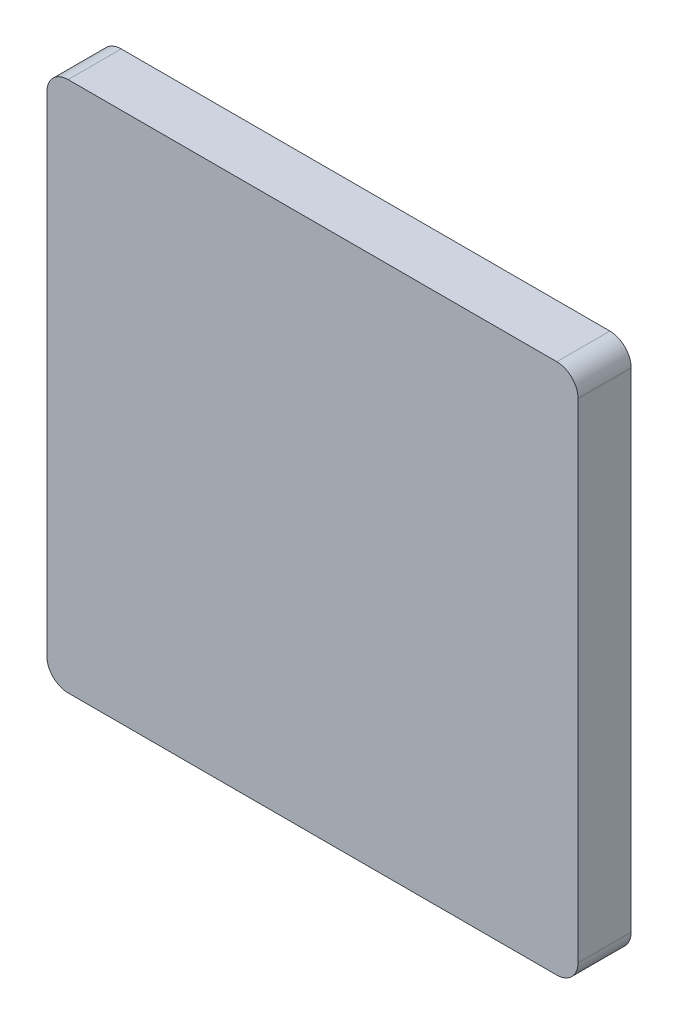
SolidWorks part; units mm, degrees
material "Q235"
ref_plane "Front Plane" through (0, 0, 0) normal (0, 0, 1) x (1, 0, 0)
ref_plane "Top Plane" through (0, 0, 0) normal (0, 1, 0) x (1, 0, 0)
ref_plane "Right Plane" through (0, 0, 0) normal (1, 0, 0) x (0, 0, -1)
sketch "Sketch1" plane through (0, 0, 0) normal (0, 0, 1) x (1, 0, 0)
  line L1 (-30, -30) -> (30, -30)
  line L2 (-30, -30) -> (-30, 30)
  line L3 (-30, 30) -> (30, 30)
  line L4 (30, -30) -> (30, 30)
  line L5 (-30, -30) -> (30, 30) construction
  line L6 (-30, 30) -> (30, -30) construction
  line L7 (-26, -26) -> (26, -26)
  line L8 (-26, -26) -> (-26, 26)
  line L9 (-26, 26) -> (26, 26)
  line L10 (26, -26) -> (26, 26)
  line L11 (-26, -26) -> (26, 26) construction
  line L12 (-26, 26) -> (26, -26) construction
  point P0 (0, 0)
  point P5 (0, 0)
  dimension "D1" = 4
  dimension "D2" = 60
  dimension "D3" = 60
extrude "Boss-Extrude1" add sketch "Sketch1" along normal blind 400
fillet "Fillet1" radius 6 4 edges at (30, -30, 200) (-30, -30, 200) (30, 30, 200) (-30, 30, 200)
fillet "Fillet2" radius 3 4 edges at (26, -26, 200) (-26, -26, 200) (26, 26, 200) (-26, 26, 200)
sketch "Sketch2" plane through (0, 0, 0) normal (0, 0, -1) x (-1, 0, 0)
  line L0 (-26, -23) -> (-26, 23) construction
  line L1 (-23, 26) -> (23, 26) construction
  line L2 (26, 23) -> (26, -23) construction
  line L3 (23, -26) -> (-23, -26) construction
  line L4 (-26, -23) -> (-26, 23) construction
  line L5 (-23, 26) -> (23, 26) construction
  line L6 (26, 23) -> (26, -23) construction
  line L7 (23, -26) -> (-23, -26) construction
  line L8 (25, 23) -> (25, -23)
  line L9 (-23, 25) -> (23, 25)
  line L10 (-25, -23) -> (-25, 23)
  line L11 (23, -25) -> (-23, -25)
  arc A0 (-26, -23) -> (-23, -26) centre (-23, -23) ccw construction
  arc A1 (-23, 26) -> (-26, 23) centre (-23, 23) ccw construction
  arc A2 (26, 23) -> (23, 26) centre (23, 23) ccw construction
  arc A3 (23, -26) -> (26, -23) centre (23, -23) ccw construction
  arc A4 (-26, -23) -> (-23, -26) centre (-23, -23) ccw construction
  arc A5 (-23, 26) -> (-26, 23) centre (-23, 23) ccw construction
  arc A6 (26, 23) -> (23, 26) centre (23, 23) ccw construction
  arc A7 (23, -26) -> (26, -23) centre (23, -23) ccw construction
  arc A8 (23, -25) -> (25, -23) centre (23, -23) ccw
  arc A9 (25, 23) -> (23, 25) centre (23, 23) ccw
  arc A10 (-23, 25) -> (-25, 23) centre (-23, 23) ccw
  arc A11 (-25, -23) -> (-23, -25) centre (-23, -23) ccw
  dimension "D1" = 1
extrude "Boss-Extrude2" add sketch "Sketch2" along normal blind 5 separate body
sketch "Sketch4" plane through (0, 0, 0) normal (0, 0, -1) x (-1, 0, 0)
  line L0 (26, 23) -> (26, -23) construction
  line L1 (-23, 26) -> (23, 26) construction
  line L2 (-26, -23) -> (-26, 23) construction
  line L3 (23, -26) -> (-23, -26) construction
  line L4 (-30, 24) -> (-30, -24)
  line L5 (-24, -30) -> (24, -30)
  line L6 (30, -24) -> (30, 24)
  line L7 (24, 30) -> (-24, 30)
  line L8 (-30, 24) -> (-30, -24)
  line L9 (-24, -30) -> (24, -30)
  line L10 (30, -24) -> (30, 24)
  line L11 (24, 30) -> (-24, 30)
  line L12 (26, 23) -> (26, -23)
  line L13 (-23, 26) -> (23, 26)
  line L14 (-26, -23) -> (-26, 23)
  line L15 (23, -26) -> (-23, -26)
  arc A0 (26, 23) -> (23, 26) centre (23, 23) ccw construction
  arc A1 (-23, 26) -> (-26, 23) centre (-23, 23) ccw construction
  arc A2 (-26, -23) -> (-23, -26) centre (-23, -23) ccw construction
  arc A3 (23, -26) -> (26, -23) centre (23, -23) ccw construction
  arc A4 (-30, -24) -> (-24, -30) centre (-24, -24) ccw
  arc A5 (24, -30) -> (30, -24) centre (24, -24) ccw
  arc A6 (30, 24) -> (24, 30) centre (24, 24) ccw
  arc A7 (-24, 30) -> (-30, 24) centre (-24, 24) ccw
  arc A8 (-30, -24) -> (-24, -30) centre (-24, -24) ccw
  arc A9 (24, -30) -> (30, -24) centre (24, -24) ccw
  arc A10 (30, 24) -> (24, 30) centre (24, 24) ccw
  arc A11 (-24, 30) -> (-30, 24) centre (-24, 24) ccw
  arc A12 (26, 23) -> (23, 26) centre (23, 23) ccw
  arc A13 (-23, 26) -> (-26, 23) centre (-23, 23) ccw
  arc A14 (-26, -23) -> (-23, -26) centre (-23, -23) ccw
  arc A15 (23, -26) -> (26, -23) centre (23, -23) ccw
  dimension "D1" = 0
extrude "Cut-Extrude1" cut sketch "Sketch4" against normal through all contours L8 A8 L9 A9 L10 A10 L11 A11
